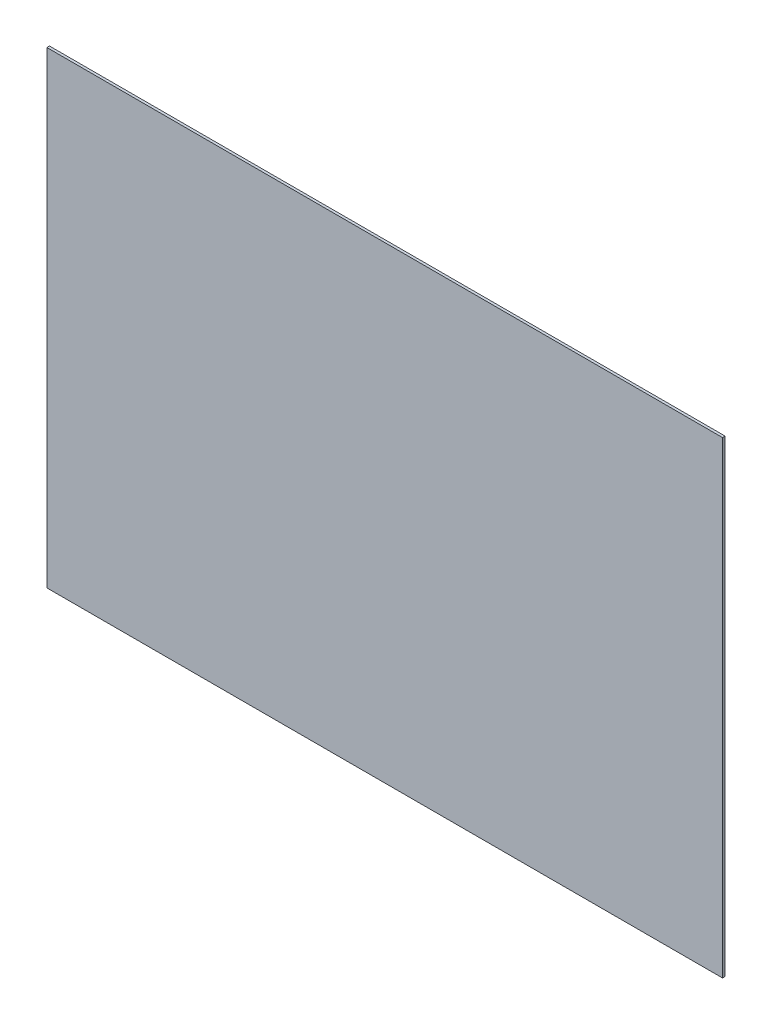
SolidWorks part; units mm, degrees
material "有机玻璃 (PMMA)"
ref_plane "前视" through (0, 0, 0) normal (0, 0, 1) x (1, 0, 0)
ref_plane "上视" through (0, 0, 0) normal (0, 1, 0) x (1, 0, 0)
ref_plane "右视" through (0, 0, 0) normal (1, 0, 0) x (0, 0, -1)
sketch "草图1" plane through (0, 0, 0) normal (0, 0, 1) x (1, 0, 0)
  line L1 (524, -363) -> (-524, -363)
  line L2 (524, -363) -> (524, 363)
  line L3 (524, 363) -> (-524, 363)
  line L4 (-524, -363) -> (-524, 363)
  line L5 (524, -363) -> (-524, 363) construction
  line L6 (524, 363) -> (-524, -363) construction
  point P0 (0, 0)
  dimension "D1" = 1048
  dimension "D2" = 726
extrude "凸台-拉伸1" add sketch "草图1" along normal blind 4
